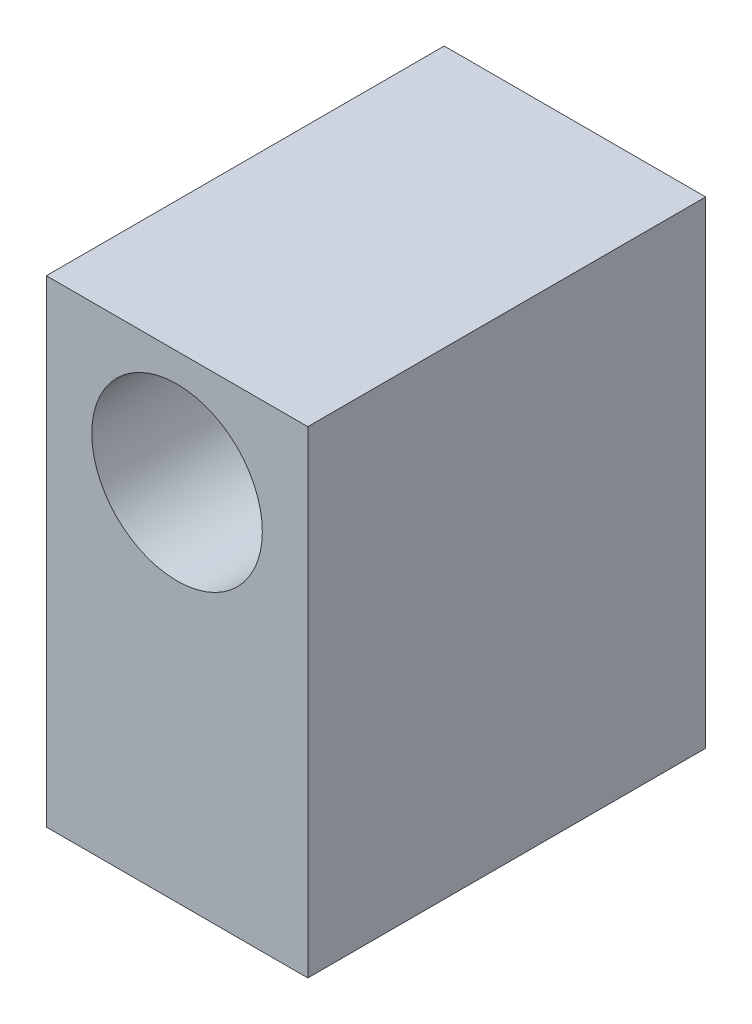
from build123d import *

# Parameters (mm, degrees)
SKETCH_1_W          = 23
SKETCH_1_H          = 42
SKETCH_1_R          = 7.5
EXTRUDE_1_DEPTH     = 35
SKETCH_2_R          = 2.1
CUT_EXTRUDE_1_DEPTH = 11.5
SKETCH_3_R          = 2.5
CUT_EXTRUDE_2_DEPTH = 10


with BuildPart() as part:
    # 草图1 → 凸台-拉伸1 (new body)
    with BuildSketch(Plane.XY):
        with Locations((1.112903226, 1.756048387)):
            Rectangle(SKETCH_1_W, SKETCH_1_H)
        with Locations((1.112903226, 12.756048387)):
            Circle(SKETCH_1_R, mode=Mode.SUBTRACT)
    extrude(amount=EXTRUDE_1_DEPTH)

    # 草图2 → 切除-拉伸1 (cut)
    with BuildSketch(Plane.XZ.offset(19.243951613)):
        with Locations(Location((1.112903226, 27, 0), (0, 0, 270))):
            Circle(SKETCH_2_R)
        with Locations(Location((1.112903226, 8, 0), (0, 0, 270))):
            Circle(SKETCH_2_R)
    extrude(amount=-CUT_EXTRUDE_1_DEPTH, mode=Mode.SUBTRACT)

    # 草图3 → 切除-拉伸2 (cut)
    with BuildSketch(Plane.XZ.offset(19.243951613)):
        with Locations(Location((1.112903226, 27, 0), (0, 0, 270))):
            Circle(SKETCH_3_R)
        with Locations(Location((1.112903226, 8, 0), (0, 0, 270))):
            Circle(SKETCH_3_R)
    extrude(amount=-CUT_EXTRUDE_2_DEPTH, mode=Mode.SUBTRACT)


solid = part.part
